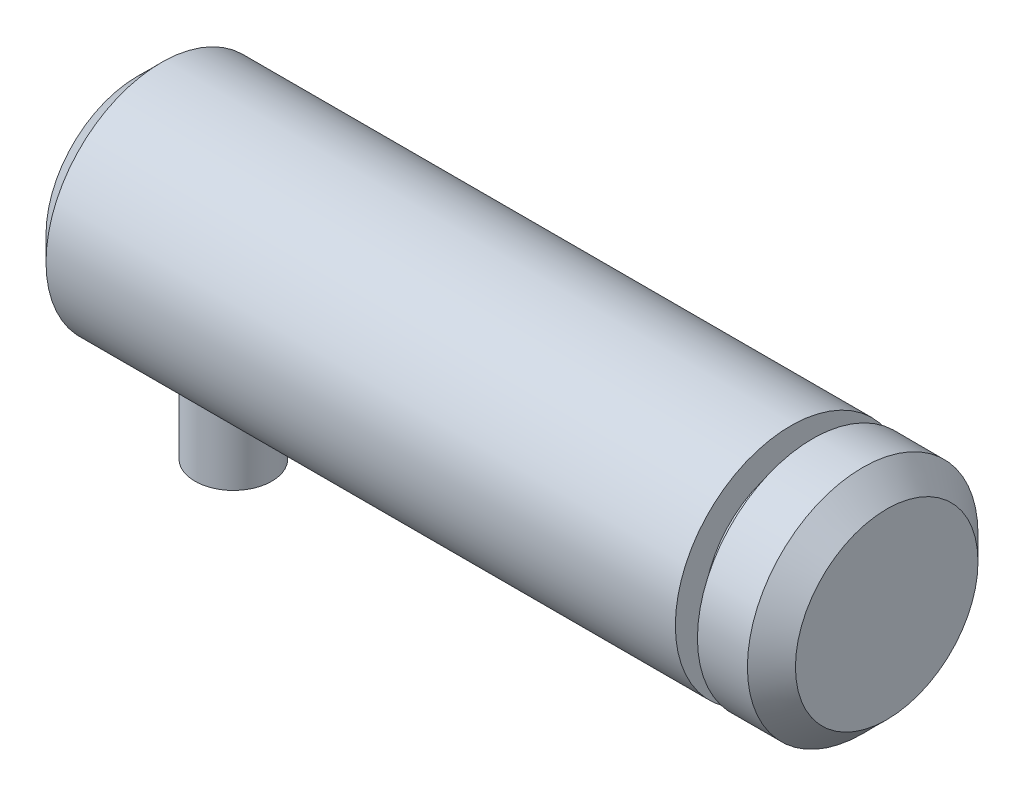
from build123d import *

# Parameters (mm, degrees)
SKETCH_2_W     = 2
SKETCH_2_H     = 4.343145751
CHAMFER_1_SIZE = 1.25


with BuildPart() as part:
    # 草图1 → 旋转1 (revolve)
    with BuildSketch(Plane(origin=(0, 0, 0), x_dir=(-1, 0, 0), z_dir=(0, 0, -1)), mode=Mode.PRIVATE) as revolve_1_sk:
        Polygon((-19.5, 6), (-19.5, 0), (19.5, 0), (19.5, 6), (-14.5, 6), (-14.5, 4.5), (-15.65, 4.5), (-15.65, 6), align=None)
    revolve(revolve_1_sk.sketch.rotate(Axis((19.5, 0, 0), (-1, 0, 0)), 270), axis=Axis((19.5, 0, 0), (-1, 0, 0)))

    # 草图2 → 旋转2 (revolve)
    with BuildSketch(Plane(origin=(-14.5, 0, 0), x_dir=(0, 0, -1), z_dir=(1, 0, 0))):
        with Locations((1, -7.828427125)):
            Rectangle(SKETCH_2_W, SKETCH_2_H)
    revolve(axis=Axis((-14.5, -5.656854249, 0), (0, -1, 0)))

    # 倒角1
    chamfer_1_edges = [part.edges().sort_by_distance(p)[0] for p in [
        (19.5, 0, -6),
        (-19.5, 0, -6),
    ]]
    chamfer(chamfer_1_edges, length=CHAMFER_1_SIZE)


solid = part.part
